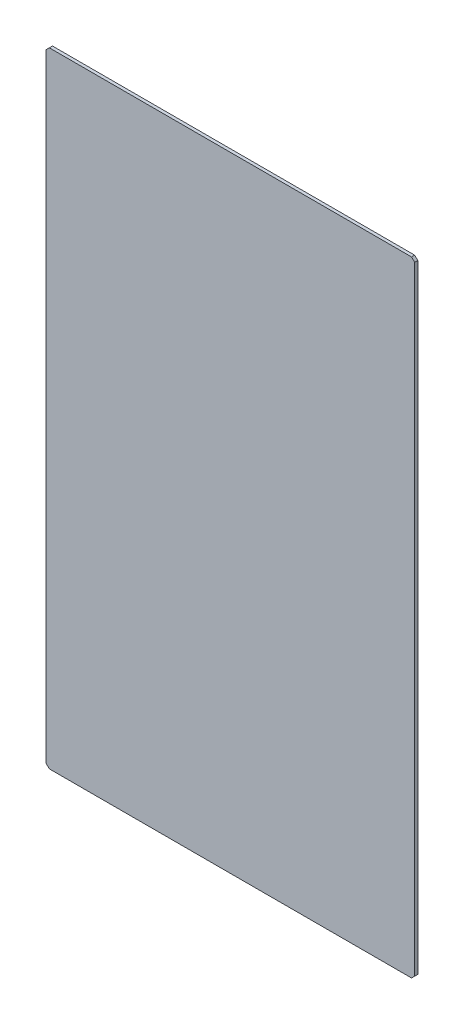
SolidWorks part; units mm, degrees
material "丙烯酸 (中高冲力)"
ref_plane "前视基准面" through (0, 0, 0) normal (0, 0, 1) x (1, 0, 0)
ref_plane "上视基准面" through (0, 0, 0) normal (0, 1, 0) x (1, 0, 0)
ref_plane "右视基准面" through (0, 0, 0) normal (1, 0, 0) x (0, 0, -1)
sketch "草图1" plane through (0, 0, 0) normal (0, 0, 1) x (1, 0, 0)
  line L0 (-295, 500) -> (295, -500) construction
  line L1 (-295, 500) -> (295, 500)
  line L2 (-295, 500) -> (-295, -500)
  line L3 (-295, -500) -> (295, -500)
  line L4 (295, 500) -> (295, -500)
  dimension "D1" = 590
  dimension "D2" = 1000
extrude "拉伸1" add sketch "草图1" along normal blind 5
chamfer "倒角1" distance 5 angle 45 4 edges at (-295, -500, 2.5) (295, -500, 2.5) (295, 500, 2.5) (-295, 500, 2.5)
